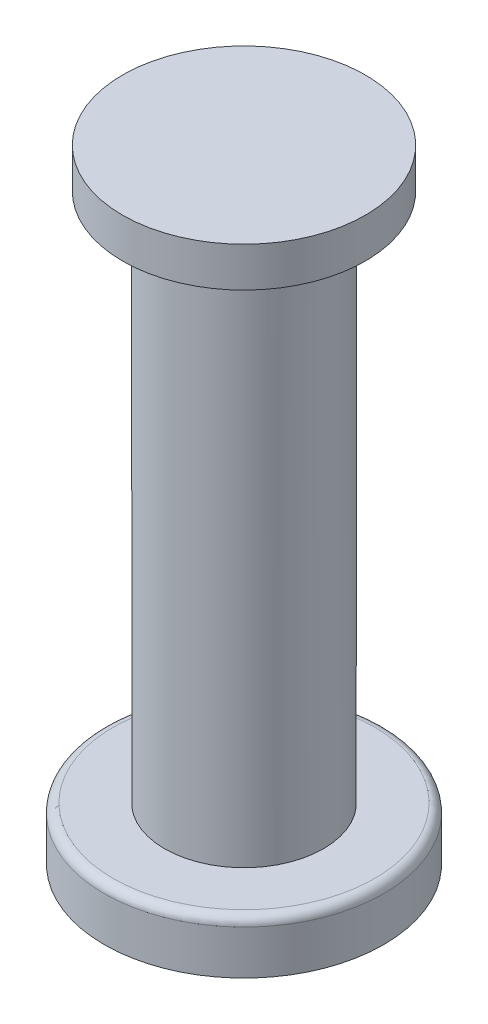
from build123d import *

# Parameters (mm, degrees)
SKETCH1_R           = 137.5
BOSS_EXTRUDE1_DEPTH = 45
SKETCH2_R           = 90
BOSS_EXTRUDE2_DEPTH = 600
SKETCH3_R           = 158.18220737
BOSS_EXTRUDE3_DEPTH = 60
FILLET1_R           = 10


with BuildPart() as part:
    # Sketch1 → Boss-Extrude1 (new body)
    with BuildSketch(Plane(origin=(0, 0, 0), x_dir=(1, 0, 0), z_dir=(0, 1, 0))):
        with Locations(Location((0, 0, 0), (0, 0, 270))):
            Circle(SKETCH1_R)
    extrude(amount=BOSS_EXTRUDE1_DEPTH)

    # Sketch2 → Boss-Extrude2 (add)
    with BuildSketch(Plane.XZ):
        with Locations(Location((0, 0, 0), (0, 0, 90))):
            Circle(SKETCH2_R)
    extrude(amount=BOSS_EXTRUDE2_DEPTH)

    # Sketch3 → Boss-Extrude3 (add)
    with BuildSketch(Plane.XZ.offset(600)):
        with Locations(Location((0, 0, 0), (0, 0, 270))):
            Circle(SKETCH3_R)
    extrude(amount=BOSS_EXTRUDE3_DEPTH)

    # Fillet1
    fillet1_edges = [part.edges().sort_by_distance(p)[0] for p in [
        (0, -600, 158.18220737),
    ]]
    fillet(fillet1_edges, radius=FILLET1_R)


solid = part.part
